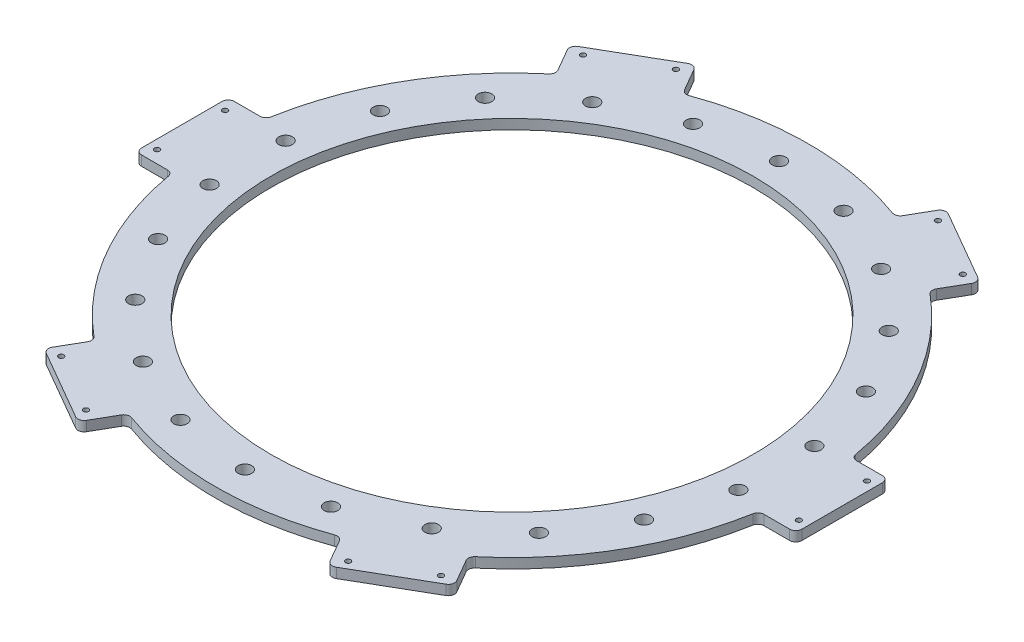
from build123d import *

# Parameters (mm, degrees)
SKETCH2_R                  = 480
SKETCH2_R_2                = 390
BOSS_EXTRUDE1_DEPTH        = 16
FILLET1_R                  = 10
F_22_0_22_DIAMETER_HOLE1_D = 22
M10_TAPPED_HOLE1_D         = 8.5


with BuildPart() as part:
    # Sketch2 → Boss-Extrude1 (new body)
    # profile 1 of 7: a face of its own
    with BuildSketch(Plane(origin=(0, 0, 0), x_dir=(1, 0, 0), z_dir=(0, 1, 0))):
        Circle(SKETCH2_R)
        with Locations(Location((0, 0, 0), (0, 0, 270))):
            Circle(SKETCH2_R_2, mode=Mode.SUBTRACT)
    # profile 2 of 7: a face of its own
    with BuildSketch(Plane(origin=(0, 0, 0), x_dir=(1, 0, 0), z_dir=(0, 1, 0))):
        with BuildLine():
            Line((-326.951905284, 416.297311583), (-302.004114723, 373.086470795))
            ThreePointArc((-302.004114723, 373.086470795), (-240, 415.692193817), (-172.100304155, 448.086470795))
            Line((-172.100304155, 448.086470795), (-197.048094716, 491.297311583))
            ThreePointArc((-197.048094716, 491.297311583), (-203.120158303, 495.956569846), (-210.708348754, 494.957565621))
            Line((-210.708348754, 494.957565621), (-323.291651246, 429.957565621))
            ThreePointArc((-323.291651246, 429.957565621), (-327.950909509, 423.885502034), (-326.951905284, 416.297311583))
        make_face()
    # profile 3 of 7: a face of its own
    with BuildSketch(Plane(origin=(0, 0, 0), x_dir=(1, 0, 0), z_dir=(0, 1, 0))):
        with BuildLine():
            ThreePointArc((-474.104418878, -75), (-480, 0), (-474.104418878, 75))
            Line((-474.104418878, 75), (-524, 75))
            ThreePointArc((-524, 75), (-531.071067812, 72.071067812), (-534, 65))
            Line((-534, 65), (-534, -65))
            ThreePointArc((-534, -65), (-531.071067812, -72.071067812), (-524, -75))
            Line((-524, -75), (-474.104418878, -75))
        make_face()
    # profile 4 of 7: a face of its own
    with BuildSketch(Plane(origin=(0, 0, 0), x_dir=(1, 0, 0), z_dir=(0, 1, 0))):
        with BuildLine():
            ThreePointArc((-172.100304155, -448.086470795), (-240, -415.692193817), (-302.004114723, -373.086470795))
            Line((-302.004114723, -373.086470795), (-326.951905284, -416.297311583))
            ThreePointArc((-326.951905284, -416.297311583), (-327.950909509, -423.885502034), (-323.291651246, -429.957565621))
            Line((-323.291651246, -429.957565621), (-210.708348754, -494.957565621))
            ThreePointArc((-210.708348754, -494.957565621), (-203.120158303, -495.956569846), (-197.048094716, -491.297311583))
            Line((-197.048094716, -491.297311583), (-172.100304155, -448.086470795))
        make_face()
    # profile 5 of 7: a face of its own
    with BuildSketch(Plane(origin=(0, 0, 0), x_dir=(1, 0, 0), z_dir=(0, 1, 0))):
        with BuildLine():
            ThreePointArc((302.004114723, -373.086470795), (240, -415.692193817), (172.100304155, -448.086470795))
            Line((172.100304155, -448.086470795), (197.048094716, -491.297311583))
            ThreePointArc((197.048094716, -491.297311583), (203.120158303, -495.956569846), (210.708348754, -494.957565621))
            Line((210.708348754, -494.957565621), (323.291651246, -429.957565621))
            ThreePointArc((323.291651246, -429.957565621), (327.950909509, -423.885502034), (326.951905284, -416.297311583))
            Line((326.951905284, -416.297311583), (302.004114723, -373.086470795))
        make_face()
    # profile 6 of 7: a face of its own
    with BuildSketch(Plane(origin=(0, 0, 0), x_dir=(1, 0, 0), z_dir=(0, 1, 0))):
        with BuildLine():
            Line((524, 75), (474.104418878, 75))
            ThreePointArc((474.104418878, 75), (478.523834862, 37.615681161), (480, 0))
            ThreePointArc((480, 0), (478.523834862, -37.615681161), (474.104418878, -75))
            Line((474.104418878, -75), (524, -75))
            ThreePointArc((524, -75), (531.071067812, -72.071067812), (534, -65))
            Line((534, -65), (534, 65))
            ThreePointArc((534, 65), (531.071067812, 72.071067812), (524, 75))
        make_face()
    # profile 7 of 7: a face of its own
    with BuildSketch(Plane(origin=(0, 0, 0), x_dir=(1, 0, 0), z_dir=(0, 1, 0))):
        with BuildLine():
            Line((197.048094716, 491.297311583), (172.100304155, 448.086470795))
            ThreePointArc((172.100304155, 448.086470795), (240, 415.692193817), (302.004114723, 373.086470795))
            Line((302.004114723, 373.086470795), (326.951905284, 416.297311583))
            ThreePointArc((326.951905284, 416.297311583), (327.950909509, 423.885502034), (323.291651246, 429.957565621))
            Line((323.291651246, 429.957565621), (210.708348754, 494.957565621))
            ThreePointArc((210.708348754, 494.957565621), (203.120158303, 495.956569846), (197.048094716, 491.297311583))
        make_face()
    extrude(amount=BOSS_EXTRUDE1_DEPTH)

    # Fillet1
    fillet1_edges = [part.edges().sort_by_distance(p)[0] for p in [
        (-172.100304155, 8, 448.086470795),
        (-302.004114723, 8, 373.086470795),
        (-474.104418878, 8, 75),
        (-474.104418878, 8, -75),
        (-302.004114723, 8, -373.086470795),
        (-172.100304155, 8, -448.086470795),
        (172.100304155, 8, -448.086470795),
        (302.004114723, 8, -373.086470795),
        (474.104418878, 8, -75),
        (474.104418878, 8, 75),
        (302.004114723, 8, 373.086470795),
        (172.100304155, 8, 448.086470795),
    ]]
    fillet(fillet1_edges, radius=FILLET1_R)

    # Ø22.0 (22) Diameter Hole1 (through all)
    with Locations(Plane(origin=(0, 16, 0), x_dir=(1, 0, 0), z_dir=(0, 1, 0))):
        with Locations((0, 432), (121.708464555, 414.500964601), (233.556833141, 363.421526183), (326.483816121, 282.899837064), (392.961021993, 179.459285617), (427.602862893, 61.480010134), (427.602862893, -61.480010134), (392.961021993, -179.459285617), (326.483816121, -282.899837064), (233.556833141, -363.421526183), (121.708464555, -414.500964601), (0, -432), (-121.708464555, -414.500964601), (-233.556833141, -363.421526183), (-326.483816121, -282.899837064), (-392.961021993, -179.459285617), (-427.602862893, -61.480010134), (-427.602862893, 61.480010134), (-392.961021993, 179.459285617), (-326.483816121, 282.899837064), (-233.556833141, 363.421526183), (-121.708464555, 414.500964601)):
            Hole(F_22_0_22_DIAMETER_HOLE1_D / 2)

    # M10 Tapped Hole1 (through all)
    with Locations(Plane(origin=(0, 16, 0), x_dir=(1, 0, 0), z_dir=(0, 1, 0))):
        with Locations((-519.094403746, 55), (-519.094403746, -55), (-211.915804665, 477.048940606), (-307.178599081, 422.048940606), (307.178599081, 422.048940606), (211.915804665, 477.048940606), (519.094403746, -55), (519.094403746, 55), (211.915804665, -477.048940606), (307.178599081, -422.048940606), (-307.178599081, -422.048940606), (-211.915804665, -477.048940606)):
            Hole(M10_TAPPED_HOLE1_D / 2)


solid = part.part
